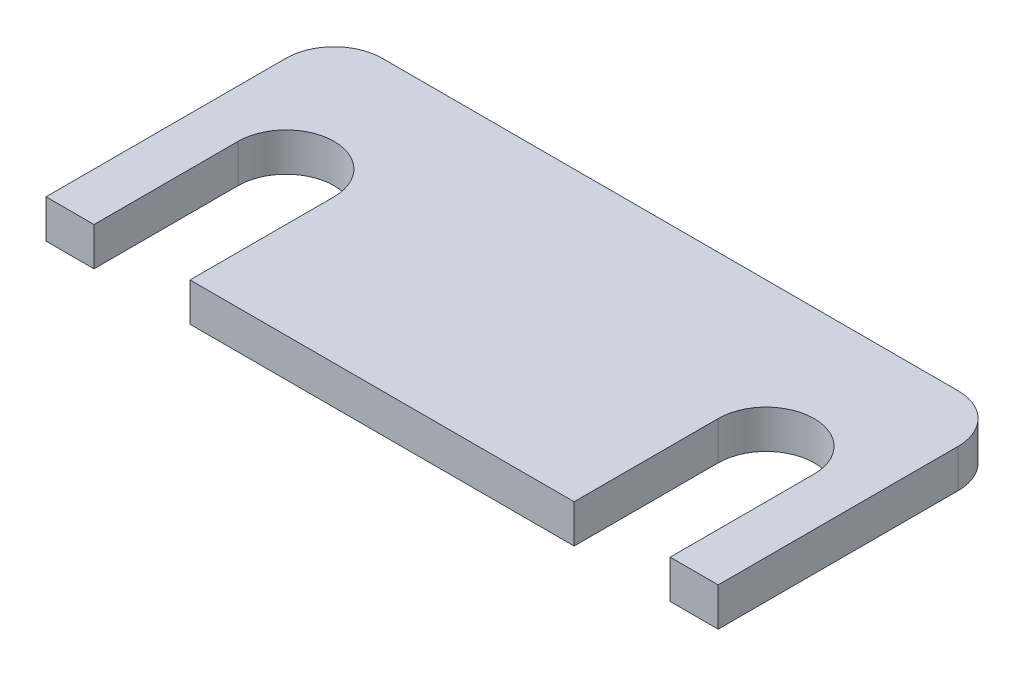
SolidWorks part; units mm, degrees
material "A3"
ref_plane "前视基准面" through (0, 0, 0) normal (0, 0, 1) x (1, 0, 0)
ref_plane "上视基准面" through (0, 0, 0) normal (0, 1, 0) x (1, 0, 0)
ref_plane "右视基准面" through (0, 0, 0) normal (1, 0, 0) x (0, 0, -1)
sketch "草图1" plane through (0, 0, 0) normal (0, 1, 0) x (1, 0, 0)
  line L0 (0, 0) -> (0, 30) construction
  line L1 (30, 30) -> (-30, 30)
  line L2 (-35, 25) -> (-35, 0)
  line L3 (-35, 0) -> (-30, 0)
  line L4 (-30, 0) -> (-30, 15)
  line L5 (-30, 15) -> (-20, 15) construction
  line L6 (-20, 15) -> (-20, 0)
  line L7 (-20, 0) -> (20, 0)
  line L8 (30, 15) -> (20, 15) construction
  line L9 (20, 15) -> (20, 0)
  line L10 (30, 0) -> (30, 15)
  line L11 (35, 0) -> (30, 0)
  line L12 (35, 25) -> (35, 0)
  arc A0 (-20, 15) -> (-30, 15) centre (-25, 15) ccw
  arc A1 (-30, 30) -> (-35, 25) centre (-30, 25) ccw
  arc A2 (30, 30) -> (35, 25) centre (30, 25) cw
  arc A3 (20, 15) -> (30, 15) centre (25, 15) cw
  point P6 (-25, 15)
  point P13 (-35, 30)
  point P23 (35, 30)
  dimension "D6" = 5
  dimension "D1" = 70
  dimension "D2" = 30
  dimension "D3" = 15
  dimension "D4" = 10
  dimension "D5" = 50
extrude "凸台-拉伸1" add sketch "草图1" along normal blind 4
